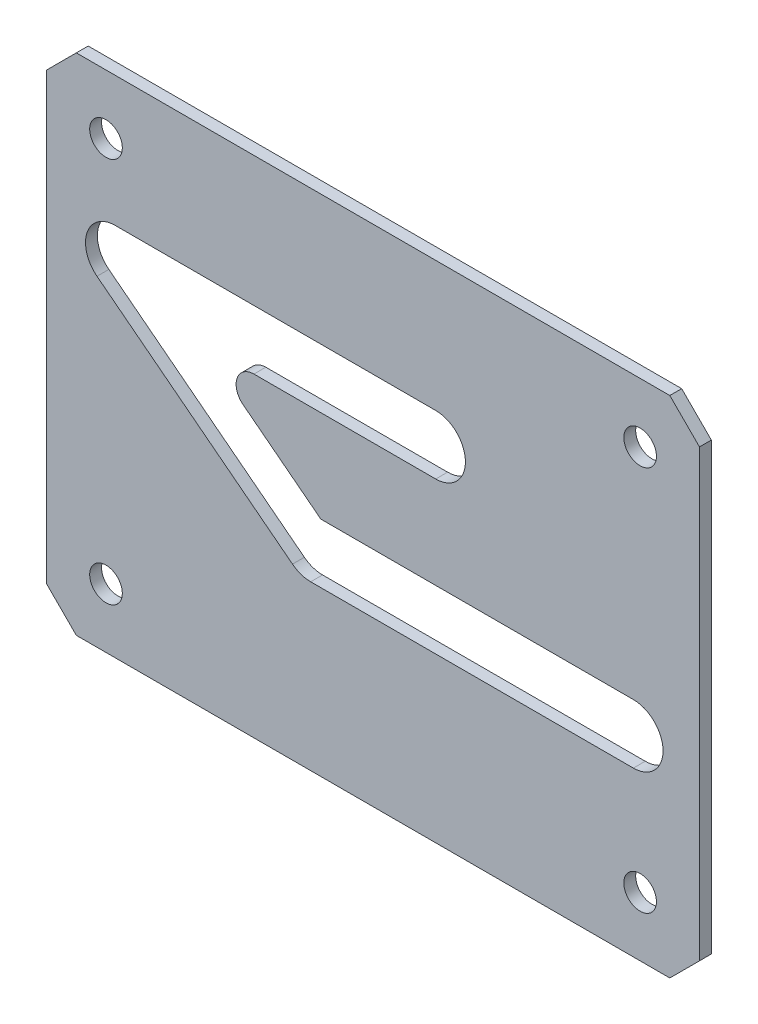
SolidWorks part; units mm, degrees
material "AL6061"
ref_plane "主视基准图" through (0, 0, 0) normal (0, 0, 1) x (1, 0, 0)
ref_plane "上视基准图" through (0, 0, 0) normal (0, 1, 0) x (1, 0, 0)
ref_plane "右视基准图" through (0, 0, 0) normal (1, 0, 0) x (0, 0, -1)
sketch "Model" plane through (0, 0, 0) normal (0, 0, 1) x (1, 0, 0)
  line L0 (186.507, 241.5119) -> (58.9109, 92.8097)
  line L3 (-18.5, 320) -> (-18.5, 197.0297) construction
  line L4 (-83.5, 335) -> (-83.5, 10)
  line L5 (-73.5, 0) -> (56.5, 0)
  line L6 (56.5, 0) -> (56.5, 86.2977)
  line L7 (59.5, 335) -> (-83.5, 335)
  line L9 (69.5, 345) -> (69.5, 435)
  line L10 (259.5, 245) -> (194.0961, 245)
  line L11 (269.5, 425) -> (269.5, 255)
  line L12 (69.5, 435) -> (259.5, 435)
  arc A0 (56.5, 86.2977) -> (58.9109, 92.8097) centre (66.5, 86.2977) cw
  arc A1 (269.5, 425) -> (259.5, 435) centre (259.5, 425) ccw
  arc A2 (186.507, 241.5119) -> (194.0961, 245) centre (194.0961, 235) cw
  arc A4 (-83.5, 10) -> (-73.5, 0) centre (-73.5, 10) ccw
  arc A5 (269.5, 255) -> (259.5, 245) centre (259.5, 255) cw
  arc A6 (69.5, 345) -> (59.5, 335) centre (59.5, 345) cw
  point P9 (56.5, 90)
  point P13 (189.5, 245)
  dimension "D1" = 200
  dimension "D8" = 10
  dimension "D9" = 435
  dimension "D10" = 10
  dimension "D11" = 10
  dimension "D12" = 10
  dimension "D2" = 190
  dimension "D3" = 213
  dimension "D4" = 335
  dimension "D5" = 140
  dimension "D6" = 80
  dimension "D7" = 90
extrude "凸台-拉伸1" add sketch "Model" along normal mid plane 2
hole_wizard "M6 六角凹头螺钉的柱形沉头孔1" positions "草图5" profile "草图4" counterbore size "M6" standard "Iso" end condition through all
sketch "草图5" plane through (0, 0, -1) normal (0, 0, -1) x (-1, 0, 0)
  line L1 (-9.5, 235) -> (16.5, 235) construction
  line L2 (-9.5, 235) -> (-9.5, 157) construction
  line L3 (-9.5, 157) -> (16.5, 157) construction
  line L4 (16.5, 235) -> (16.5, 157) construction
  line L5 (-9.5, 235) -> (16.5, 157) construction
  line L6 (-9.5, 157) -> (16.5, 235) construction
  line L9 (83.5, 335) -> (83.5, 10) construction
  line L10 (-259.5, 435) -> (-69.5, 435) construction
  line L11 (3.5, 196) -> (16.5, 196) construction
  point P2 (16.5, 157)
  point P97 (-9.5, 235)
  point P98 (-9.5, 157)
  point P99 (16.5, 235)
  dimension "D1" = 200
  dimension "D2" = 67
  dimension "D3" = 78
  dimension "D4" = 26
sketch "草图4" plane through (-16.5, 157, -1) normal (1, 0, 0) x (0, 1, 0)
  line L0 (0, 0) -> (0, 2)
  line L1 (0, 2) -> (3.3, 2)
  line L3 (3.3, 2) -> (3.3, 6.4)
  line L4 (3.3, 6.4) -> (5.5, 6.4)
  line L5 (5.5, 6.4) -> (5.5, 0)
  line L7 (5.5, 0) -> (0, 0)
  line L11 (0, -6.35) -> (0, 107.95) construction
  dimension "通孔孔直径" = 6.6
  dimension "通孔孔深度" = 2
  dimension "柱形沉头孔直径" = 11
  dimension "柱形沉头孔深度" = 6.4
sketch "草图27" plane through (0, 0, 1) normal (0, 0, 1) x (1, 0, 0)
  line L0 (-83.5, 335) -> (-83.5, 10) construction
  line L1 (-83.5, 435) -> (-83.5, 315)
  line L2 (259.5, 435) -> (69.5, 435) construction
  line L3 (69.5, 435) -> (-83.5, 435)
  line L4 (69.5, 435) -> (69.5, 345) construction
  line L5 (69.5, 435) -> (69.5, 315)
  line L6 (69.5, 315) -> (-83.5, 315)
  line L7 (59.5, 335) -> (-83.5, 335) construction
  dimension "D1" = 20
extrude "凸台-拉伸3" add sketch "草图27" against normal up to surface (2 mm away) up to face at (-22, 157, -1)
sketch "草图12" plane through (0, 0, 1) normal (0, 0, 1) x (1, 0, 0)
  line L1 (259.5, 435) -> (-83.5, 435) construction
  line L3 (-83.5, 435) -> (-83.5, 10) construction
  line L4 (194.0961, 245) -> (259.5, 245) construction
  circle A0 centre (-60.5, 390) radius 7 construction
  circle A1 centre (27.5, 405) radius 7 construction
  circle A2 centre (-32.5, 270) radius 7 construction
  circle A3 centre (47.5, 265) radius 7 construction
  dimension "D1" = 14
  dimension "D2" = 45
  dimension "D3" = 23
  dimension "D4" = 30
  dimension "D5" = 88
  dimension "D6" = 28
  dimension "D7" = 25
  dimension "D8" = 80
  dimension "D9" = 20
hole_wizard "M5 螺纹孔2" positions "草图14" profile "草图13" tap size "M5" standard "Iso"
sketch "草图14" plane through (0, 0, 1) normal (0, 0, 1) x (1, 0, 0)
  point P0 (-60.5, 390)
  point P3 (27.5, 405)
  point P6 (47.5, 265)
  point P9 (-32.5, 270)
sketch "草图13" plane through (-60.5, 390, 1) normal (1, 0, 0) x (0, -1, 0)
  line L0 (0, 0) -> (0, 15.2618)
  line L1 (0, 15.2618) -> (2.1, 14)
  line L2 (2.1, 14) -> (2.1, 0)
  line L5 (2.1, 0) -> (0, 0)
  line L10 (0, 15.2618) -> (-2.1, 14) construction
  line L11 (0, -6.35) -> (0, 107.95) construction
  dimension "螺纹孔钻头直径" = 4.2
  dimension "螺纹孔钻头深度" = 14
  dimension "导头角度" = 118
cosmetic thread "孔螺蚊线15" parameters "D1"=8, "D2"=5
cosmetic thread "孔螺蚊线16" parameters "D1"=8, "D2"=5
cosmetic thread "孔螺蚊线27" parameters "D1"=8, "D2"=5
cosmetic thread "孔螺蚊线28" parameters "D1"=8, "D2"=5
sketch "草图15" plane through (0, 0, 1) normal (0, 0, 1) x (1, 0, 0)
  line L0 (56.5, 0) -> (56.5, 86.2977) construction
  line L1 (56.5, 66.9972) -> (169.3898, 66.9972)
  line L2 (56.5, 66.9972) -> (56.5, 197)
  line L3 (56.5, 197) -> (169.3898, 197)
  line L4 (169.3898, 66.9972) -> (169.3898, 197)
  line L5 (-73.5, 0) -> (56.5, 0) construction
  dimension "D1" = 197
extrude "切除-拉伸1" cut sketch "草图15" against normal through all
sketch "草图16" plane through (0, 0, 1) normal (0, 0, 1) x (1, 0, 0)
  line L0 (-73.5, 0) -> (56.5, 0) construction
  line L1 (-83.5, 435) -> (-83.5, 10) construction
  circle A0 centre (-13.5, 25) radius 10
  dimension "D1" = 20
  dimension "D2" = 25
  dimension "D3" = 70
extrude "切除-拉伸2" cut sketch "草图16" against normal blind 2
sketch "草图18" plane through (0, 0, 1) normal (0, 0, 1) x (1, 0, 0)
  line L0 (269.5, 255) -> (269.5, 425) construction
  line L1 (269.5, 340) -> (297.8305, 340) construction
  circle A0 centre (244.5, 340) radius 10
  point P2 (269.5, 340)
  dimension "D1" = 20
  dimension "D2" = 25
extrude "切除-拉伸4" cut sketch "草图18" against normal blind 2
sketch "草图20" plane through (0, 0, 1) normal (0, 0, 1) x (1, 0, 0)
  line L8 (33.75, 62.375) -> (-20.67, 62.375) construction
  line L9 (33.75, 59.375) -> (-20.67, 59.375)
  line L11 (33.75, 65.375) -> (-16.4359, 65.375)
  line L12 (-20.67, 62.375) -> (-54.745, 112.48) construction
  line L13 (-23.1507, 60.6879) -> (-57.2257, 110.7929)
  line L14 (-20.5704, 67.5632) -> (-43.7642, 101.6682)
  line L15 (-54.745, 112.48) -> (-0.325, 112.48) construction
  line L16 (-54.745, 115.48) -> (-0.325, 115.48)
  line L19 (-39.6297, 109.48) -> (-0.325, 109.48)
  arc A6 (33.75, 59.375) -> (33.75, 65.375) centre (33.75, 62.375) ccw
  arc A7 (-20.5704, 67.5632) -> (-16.4359, 65.375) centre (-16.4359, 70.375) ccw
  arc A8 (-23.1507, 60.6879) -> (-20.67, 59.375) centre (-20.67, 62.375) ccw
  arc A9 (-43.7642, 101.6682) -> (-39.6297, 109.48) centre (-39.6297, 104.48) cw
  arc A10 (-54.745, 115.48) -> (-57.2257, 110.7929) centre (-54.745, 112.48) ccw
  arc A11 (-0.325, 109.48) -> (-0.325, 115.48) centre (-0.325, 112.48) ccw
  point P31 (3.54, 62.175)
  point P36 (-40.7075, 87.2275)
  dimension "D4" = 6
  dimension "D5" = 6
sketch "草图21" plane through (0, 0, 1) normal (0, 0, 1) x (1, 0, 0)
  line L1 (-65.5, 129.9275) -> (44.5, 129.9275) construction
  line L2 (-65.5, 129.9275) -> (-65.5, 44.9275) construction
  line L3 (-65.5, 44.9275) -> (44.5, 44.9275) construction
  line L4 (44.5, 129.9275) -> (44.5, 44.9275) construction
  line L5 (-83.5, 435) -> (-83.5, 10) construction
  line L6 (34.5, 413) -> (-65.5, 413) construction
  line L7 (-65.5, 413) -> (-65.5, 258) construction
  line L8 (-65.5, 258) -> (59.5, 258) construction
  line L9 (34.5, 413) -> (59.5, 258) construction
  line L10 (259.5, 435) -> (-83.5, 435) construction
  line L12 (-10.5, 129.9275) -> (-10.5, 44.9275) construction
  line L13 (-65.5, 87.4275) -> (44.5, 87.4275) construction
  line L14 (-83.5, 435) -> (-83.5, 10) construction
  line L18 (-0.325, 112.48) -> (-0.325, 62.375) construction
  line L19 (33.75, 62.375) -> (-20.67, 62.375) construction
  line L20 (-0.325, 87.4275) -> (69.9455, 87.4275) construction
  circle A0 centre (-5.5, 330) radius 2.5 construction
  circle A1 centre (-40.5, 80.9275) radius 2.5 construction
  circle A2 centre (-50.5, 59.9275) radius 2.5 construction
  circle A3 centre (38.5, 51.9275) radius 2.5 construction
  circle A4 centre (24.5, 114.9275) radius 2.5 construction
  circle A5 centre (-58.5, 122.9275) radius 2.5 construction
  circle A6 centre (-50.5, 405) radius 2.5 construction
  circle A7 centre (29.5, 358) radius 2.5 construction
  circle A8 centre (34.5, 283) radius 2.5 construction
  circle A9 centre (-50.5, 278) radius 2.5 construction
  dimension "D11" = 60
  dimension "D12" = 5
  dimension "D13" = 36
  dimension "D14" = 25
  dimension "D15" = 5
  dimension "D16" = 5
  dimension "D17" = 15
  dimension "D18" = 15
  dimension "D19" = 6
  dimension "D20" = 7
  dimension "D21" = 20
  dimension "D22" = 15
  dimension "D23" = 7
  dimension "D24" = 7
  dimension "D25" = 5
  dimension "D26" = 20
  dimension "D27" = 15
  dimension "D28" = 25
  dimension "D29" = 100
  dimension "D30" = 100
  dimension "D31" = 95
  dimension "D32" = 15
  dimension "D2" = 85
  dimension "D3" = 110
  dimension "D4" = 18
  dimension "D5" = 100
  dimension "D6" = 155
  dimension "D7" = 125
  dimension "D8" = 22
  dimension "D9" = 18
  dimension "D10" = 72
  dimension "D33" = 8
sketch "草图28" plane through (0, 0, 1) normal (0, 0, 1) x (1, 0, 0)
  line L0 (259.5, 435) -> (-83.5, 435) construction
  line L1 (76.5, 435) -> (342.7096, 435)
  line L2 (76.5, 435) -> (76.5, 180.0312)
  line L3 (76.5, 180.0312) -> (342.7096, 180.0312)
  line L4 (342.7096, 435) -> (342.7096, 180.0312)
  line L5 (-83.5, 435) -> (-83.5, 10) construction
  dimension "D1" = 160
extrude "切除-拉伸7" cut sketch "草图28" against normal through all
sketch "草图29" plane through (0, 0, 1) normal (0, 0, 1) x (1, 0, 0)
  line L0 (76.5, 435) -> (76.5, 197) construction
  line L1 (56.5, 197) -> (76.5, 197)
  line L2 (56.5, 197) -> (56.5, 0)
  line L3 (56.5, 0) -> (76.5, 0)
  line L4 (76.5, 197) -> (76.5, 0)
  line L5 (-73.5, 0) -> (56.5, 0) construction
extrude "凸台-拉伸4" add sketch "草图29" against normal up to surface (2 mm away)
sketch "草图30" plane through (0, 0, 1) normal (0, 0, 1) x (1, 0, 0)
  line L0 (76.5, 435) -> (76.5, 0) construction
  line L1 (-83.5, 435) -> (76.5, 435)
  line L2 (-83.5, 435) -> (-83.5, 463)
  line L3 (-83.5, 463) -> (76.5, 463)
  line L4 (76.5, 435) -> (76.5, 463)
  dimension "D1" = 28
extrude "凸台-拉伸5" add sketch "草图30" against normal up to surface (2 mm away)
ref_plane "基准面1" through (0, 231.5, 0) normal (0, 1, 0) x (1, 0, 0)
mirror "镜向1" about plane through (0, 231.5, 0) normal (0, 1, 0) of "切除-拉伸2"
sketch "草图31" plane through (0, 0, 1) normal (0, 0, 1) x (1, 0, 0)
  line L0 (-83.5, 463) -> (-83.5, 10) construction
  line L1 (-83.5, 140) -> (76.5, 140)
  line L2 (-83.5, 140) -> (-83.5, 463)
  line L3 (-83.5, 463) -> (76.5, 463)
  line L4 (76.5, 140) -> (76.5, 463)
  line L5 (-73.5, 0) -> (76.5, 0) construction
  dimension "D1" = 140
extrude "切除-拉伸8" cut sketch "草图31" against normal through all
sketch "草图32" plane through (0, 0, 1) normal (0, 0, 1) x (1, 0, 0)
  line L0 (44.5, 129.9275) -> (44.5, 44.9275) construction
  line L1 (76.5, 140) -> (49.5, 140)
  line L2 (76.5, 140) -> (76.5, 0)
  line L3 (76.5, 0) -> (49.5, 0)
  line L4 (49.5, 140) -> (49.5, 0)
  line L6 (-73.5, 0) -> (76.5, 0) construction
  dimension "D1" = 5
extrude "切除-拉伸9" cut sketch "草图32" against normal through all
sketch "草图33" plane through (0, 0, 1) normal (0, 0, 1) x (1, 0, 0)
  circle A1 centre (-13.5, 25) radius 10
extrude "凸台-拉伸6" add sketch "草图33" against normal up to surface (2 mm away)
sketch "草图37" plane through (0, 0, 1) normal (0, 0, 1) x (1, 0, 0)
  line L0 (-83.5, 140) -> (-83.5, 10) construction
  line L1 (49.5, 0) -> (-73.5, 0)
  line L2 (49.5, 0) -> (49.5, -20)
  line L3 (49.5, -20) -> (-83.5, -20)
  line L4 (-83.5, 10) -> (-83.5, -20)
  arc A0 (-83.5, 10) -> (-73.5, 0) centre (-73.5, 10) ccw construction
  arc A1 (-83.5, 10) -> (-73.5, 0) centre (-73.5, 10) ccw
  dimension "D1" = 20
extrude "凸台-拉伸7" add sketch "草图37" against normal up to surface (2 mm away)
sketch "草图34" plane through (0, 0, 1) normal (0, 0, 1) x (1, 0, 0)
  line L1 (-40.5, 15) -> (19.5, 15)
  line L2 (-40.5, 15) -> (-40.5, -10)
  line L3 (-40.5, -10) -> (19.5, -10)
  line L4 (19.5, 15) -> (19.5, -10)
  line L5 (-10.5, 15) -> (-10.5, -10) construction
  line L6 (-83.5, -20) -> (49.5, -20) construction
  line L7 (-83.5, 140) -> (-83.5, -20) construction
  dimension "D1" = 10
  dimension "D2" = 60
  dimension "D3" = 25
  dimension "D4" = 73
hole_wizard "M6 六角凹头螺钉的柱形沉头孔2" positions "草图36" profile "草图35" counterbore size "M6" standard "Iso" end condition through all
sketch "草图36" plane through (0, 0, 1) normal (0, 0, 1) x (1, 0, 0)
  point P0 (-40.5, -10)
  point P3 (-40.5, 15)
  point P6 (19.5, 15)
  point P8 (19.5, -10)
sketch "草图35" plane through (-40.5, -10, 1) normal (1, 0, 0) x (0, -1, 0)
  line L0 (0, 0) -> (0, 2)
  line L1 (0, 2) -> (3.3, 2)
  line L3 (3.3, 2) -> (3.3, 6.4)
  line L4 (3.3, 6.4) -> (5.5, 6.4)
  line L5 (5.5, 6.4) -> (5.5, 0)
  line L7 (5.5, 0) -> (0, 0)
  line L11 (0, -6.35) -> (0, 107.95) construction
  dimension "通孔孔直径" = 6.6
  dimension "通孔孔深度" = 2
  dimension "柱形沉头孔直径" = 11
  dimension "柱形沉头孔深度" = 6.4
sketch "草图38" plane through (0, 0, 1) normal (0, 0, 1) x (1, 0, 0)
  line L0 (-83.5, -20) -> (49.5, -20) construction
  line L1 (-83.5, 140) -> (-70.5, 140)
  line L2 (-83.5, 140) -> (-83.5, -20)
  line L3 (-83.5, -20) -> (-70.5, -20)
  line L4 (-70.5, 140) -> (-70.5, -20)
  dimension "D1" = 13
extrude "切除-拉伸10" cut sketch "草图38" against normal blind 10
sketch "草图39" plane through (0, 0, 1) normal (0, 0, 1) x (1, 0, 0)
  line L1 (-70.5, 140) -> (-120.5, 140)
  line L2 (-70.5, 140) -> (-70.5, 29.9275)
  line L3 (-70.5, 29.9275) -> (-120.5, 29.9275)
  line L4 (-120.5, 140) -> (-120.5, 29.9275)
  line L5 (-70.5, -20) -> (-70.5, 140) construction
  line L6 (-70.5, 140) -> (49.5, 140) construction
  line L7 (-65.5, 44.9275) -> (44.5, 44.9275) construction
  line L11 (49.5, 140) -> (49.5, -20) construction
  dimension "D1" = 15
  dimension "D2" = 170
extrude "凸台-拉伸8" add sketch "草图39" against normal up to surface (2 mm away) up to face at (-10.5, 60, -1)
sketch "草图40" plane through (0, 0, -1) normal (0, 0, -1) x (-1, 0, 0)
  line L0 (120.5, 29.9275) -> (70.5, 29.9275) construction
  line L1 (70.5, -20) -> (-49.5, -20)
  line L2 (70.5, -20) -> (70.5, 29.9275)
  line L3 (70.5, 29.9275) -> (-49.5, 29.9275)
  line L4 (-49.5, -20) -> (-49.5, 29.9275)
  line L5 (-49.5, 140) -> (-49.5, -20) construction
extrude "切除-拉伸11" cut sketch "草图40" against normal through all
sketch "草图41" plane through (0, 0, 1) normal (0, 0, -1) x (-1, 0, 0)
  line L0 (65.5, 87.4275) -> (-44.5, 87.4275) construction
  line L1 (87.5, 57.4275) -> (112.5, 57.4275)
  line L2 (87.5, 57.4275) -> (87.5, 117.4275)
  line L3 (87.5, 117.4275) -> (112.5, 117.4275)
  line L4 (112.5, 57.4275) -> (112.5, 117.4275)
  line L5 (87.5, 57.4275) -> (112.5, 117.4275) construction
  line L6 (87.5, 117.4275) -> (112.5, 57.4275) construction
  line L7 (120.5, 140) -> (120.5, 29.9275) construction
  point P0 (100, 87.4275)
  dimension "D1" = 8
  dimension "D2" = 25
  dimension "D3" = 60
hole_wizard "Ø5.5 (5.5) 直径孔1" positions "草图43" profile "草图42" hole size "Ø5.5" standard "Gb" end condition through all
sketch "草图43" plane through (0, 0, 1) normal (0, 0, 1) x (1, 0, 0)
  point P0 (-87.5, 57.4275)
  point P3 (-112.5, 57.4275)
  point P6 (-112.5, 117.4275)
  point P9 (-87.5, 117.4275)
sketch "草图42" plane through (-87.5, 57.4275, 1) normal (1, 0, 0) x (0, -1, 0)
  line L0 (0, 0) -> (0, 2)
  line L1 (0, 2) -> (2.75, 2)
  line L2 (2.75, 2) -> (2.75, 0)
  line L5 (2.75, 0) -> (0, 0)
  line L11 (0, -6.35) -> (0, 107.95) construction
  dimension "通孔孔直径" = 5.5
  dimension "通孔孔深度" = 2
other "移动面1" face at (-78, 29.9275, 0) parameters "D1"=7.5
other "移动面2" face at (-35.5, 140, 0) parameters "D1"=7.5
fillet "圆角4" radius 10 4 edges at (49.5, 22.4275, 0) (49.5, 147.5, 0) (-120.5, 147.5, 0) (-120.5, 22.4275, 0)
sketch "草图44" plane through (0, 0, 1) normal (0, 0, 1) x (1, 0, 0)
  line L0 (-65.5, 129.9275) -> (44.5, 129.9275) construction
  line L1 (44.5, 129.9275) -> (44.5, 44.9275) construction
  line L2 (-65.5, 44.9275) -> (44.5, 44.9275) construction
  line L3 (-65.5, 129.9275) -> (-65.5, 44.9275) construction
  line L4 (-65.5, 129.9275) -> (44.5, 129.9275)
  line L5 (44.5, 129.9275) -> (44.5, 44.9275)
  line L6 (-65.5, 44.9275) -> (44.5, 44.9275)
  line L7 (-65.5, 129.9275) -> (-65.5, 44.9275)
extrude "切除-拉伸12" cut sketch "草图44" against normal through all flip side to cut
chamfer "倒角1" distance 5 angle 45 4 edges at (-65.5, 129.9275, 0) (44.5, 129.9275, 0) (44.5, 44.9275, 0) (-65.5, 44.9275, 0)
hole_wizard "Ø5.5 (5.5) 直径孔2" positions "草图23" profile "草图22" hole size "Ø5.5" standard "Gb" end condition through all
sketch "草图23" plane through (0, 0, 1) normal (0, 0, 1) x (1, 0, 0)
  line L0 (39.5, 129.9275) -> (-60.5, 129.9275) construction
  line L1 (-65.5, 124.9275) -> (-65.5, 49.9275) construction
  point P12 (34.5, 54.9275)
  point P15 (34.5, 119.9275)
  point P18 (-55.5, 119.9275)
  point P21 (-55.5, 54.9275)
  dimension "D1" = 10
  dimension "D2" = 10
  dimension "D3" = 90
  dimension "D4" = 65
sketch "草图22" plane through (34.5, 54.9275, 1) normal (1, 0, 0) x (0, -1, 0)
  line L0 (0, 0) -> (0, 2)
  line L1 (0, 2) -> (2.75, 2)
  line L2 (2.75, 2) -> (2.75, 0)
  line L5 (2.75, 0) -> (0, 0)
  line L11 (0, -6.35) -> (0, 107.95) construction
  dimension "通孔孔直径" = 5.5
  dimension "通孔孔深度" = 2
sketch "草图45" plane through (0, 0, 1) normal (0, 0, 1) x (1, 0, 0)
  line L0 (33.36, 72.4886) -> (-21.0126, 72.4886)
  line L1 (33.36, 82.4886) -> (-19.3018, 82.4886)
  line L2 (0.06, 108.0215) -> (-53.9551, 108.0215)
  line L3 (-19.3018, 82.4886) -> (-32.4125, 92.6504)
  line L4 (-24.0756, 73.5367) -> (-57.0182, 99.0696)
  line L5 (0.06, 98.0215) -> (-30.5746, 98.0215)
  line L6 (0.06, 98.0215) -> (-39.3423, 98.0215) construction
  line L7 (-19.3018, 82.4886) -> (-39.3423, 98.0215) construction
  circle A0 centre (33.36, 77.3501) radius 4.8615 construction
  circle A3 centre (0.06, 103.1601) radius 4.8615 construction
  arc A4 (-53.9551, 108.0215) -> (-57.0182, 99.0696) centre (-53.9551, 103.0215) ccw
  arc A5 (-21.0126, 72.4886) -> (-24.0756, 73.5367) centre (-21.0126, 77.4886) cw
  arc A6 (-19.3018, 82.4886) -> (-19.3018, 82.4886) centre (-19.3018, 82.4886) cw
  arc A8 (33.36, 82.4886) -> (33.36, 72.4886) centre (33.36, 77.4886) cw
  arc A9 (0.06, 108.0215) -> (0.06, 98.0215) centre (0.06, 103.0215) cw
  arc A10 (-30.5746, 98.0215) -> (-32.4125, 92.6504) centre (-30.5746, 95.0215) ccw
  arc A11 (-39.3423, 98.0215) -> (-39.3423, 98.0215) centre (-39.3423, 98.0215) ccw construction
  dimension "D1" = 5
  dimension "D3" = 3
  dimension "D2" = 10
extrude "切除-拉伸13" cut sketch "草图45" against normal blind 10
